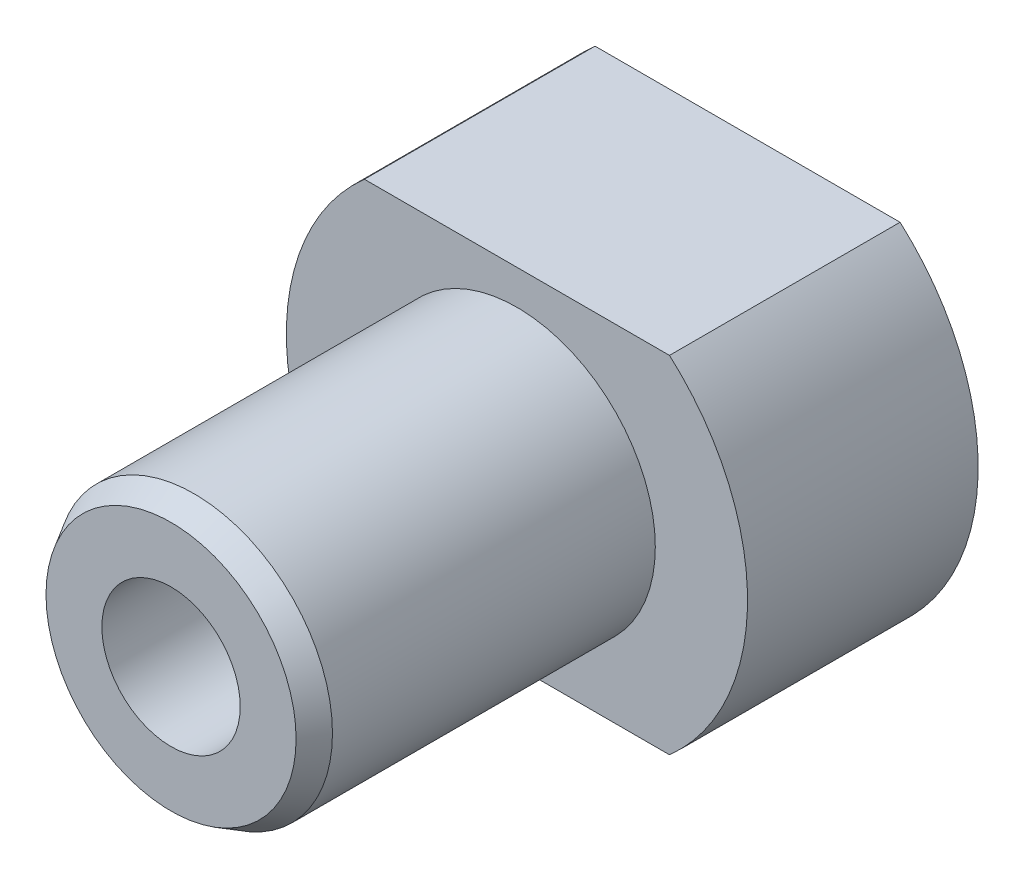
SolidWorks part; units mm, degrees
ref_plane "Front Plane" through (0, 0, 0) normal (0, 0, 1) x (1, 0, 0)
ref_plane "Top Plane" through (0, 0, 0) normal (0, 1, 0) x (1, 0, 0)
ref_plane "Right Plane" through (0, 0, 0) normal (1, 0, 0) x (0, 0, -1)
other "Configuration Table"
sketch "Sketch1" plane through (0, 0, 0) normal (0, 0, 1) x (1, 0, 0)
  circle A0 centre (0, 0) radius 3
  circle A1 centre (0, 0) radius 6
  dimension "D1" = 6
  dimension "D2" = 12
extrude "Boss-Extrude1" add sketch "Sketch1" along normal blind 15
cosmetic thread "Cosmetic Thread1" parameters "D1"=15, "D2"=11
chamfer "Chamfer1" distance 1 angle 30 1 edges at (6, 0, 15)
sketch "Sketch2" plane through (0, 0, 0) normal (0, 0, -1) x (-1, 0, 0)
  circle A0 centre (0, 0) radius 3
  circle A1 centre (0, 0) radius 10
  dimension "D1" = 20
extrude "Boss-Extrude2" add sketch "Sketch2" along normal blind 10
sketch "Sketch3" plane through (0, 0, -10) normal (0, 0, -1) x (-1, 0, 0)
  line L0 (-12.4326, 7.5) -> (-12.4326, 16.9913)
  line L1 (-12.4326, 7.5) -> (12.4326, 7.5)
  line L3 (-12.4326, -7.5) -> (12.4326, -7.5)
  line L5 (-12.4326, 7.5) -> (12.4326, -7.5) construction
  line L6 (-12.4326, -7.5) -> (12.4326, 7.5) construction
  line L7 (-12.4326, 16.9913) -> (16.5144, 13.7758)
  line L8 (16.5144, 13.7758) -> (12.4326, 7.5)
  line L9 (12.4326, -7.5) -> (9.8796, -18.9801)
  line L10 (9.8796, -18.9801) -> (-12.4326, -18.2423)
  line L11 (-12.4326, -18.2423) -> (-12.4326, -7.5)
  point P0 (0, 0)
  dimension "D1" = 15
extrude "Cut-Extrude1" cut sketch "Sketch3" against normal through all
